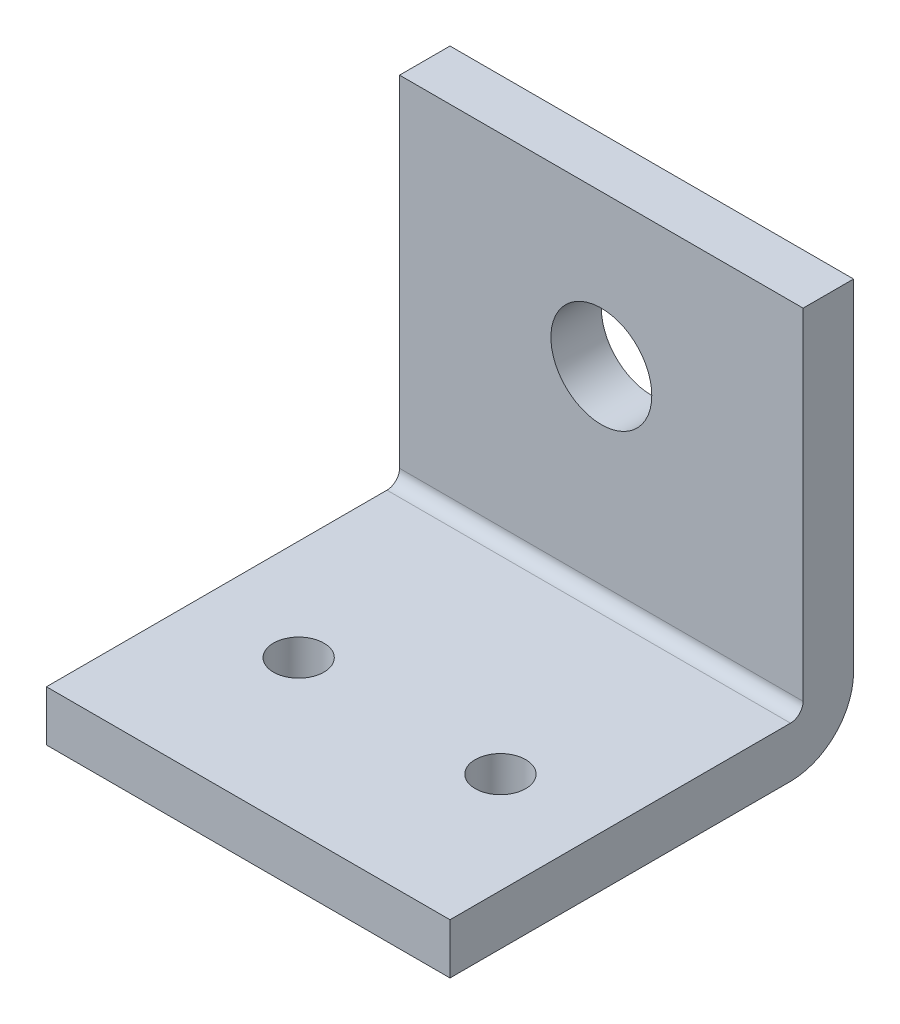
SolidWorks part; units mm, degrees
ref_plane "Front Plane" through (0, 0, 0) normal (0, 0, 1) x (1, 0, 0)
ref_plane "Top Plane" through (0, 0, 0) normal (0, 1, 0) x (1, 0, 0)
ref_plane "Right Plane" through (0, 0, 0) normal (1, 0, 0) x (0, 0, -1)
sketch "Sketch1" plane through (0, 0, 0) normal (1, 0, 0) x (0, 0, -1)
  line L0 (11.8056, 25.625) -> (11.8056, -8.125)
  line L1 (10.5556, -9.375) -> (-23.1944, -9.375)
  line L2 (-23.1944, -9.375) -> (-23.1944, -14.375)
  line L3 (-23.1944, -14.375) -> (10.5556, -14.375)
  line L4 (16.8056, -8.125) -> (16.8056, 25.625)
  line L5 (16.8056, 25.625) -> (11.8056, 25.625)
  arc A0 (16.8056, -8.125) -> (10.5556, -14.375) centre (10.5556, -8.125) cw
  arc A1 (11.8056, -8.125) -> (10.5556, -9.375) centre (10.5556, -8.125) cw
  point P8 (16.8056, -14.375)
  dimension "D5" = 6.25
  dimension "D6" = 1.25
  dimension "D1" = 5
  dimension "D2" = 5
  dimension "D3" = 40
  dimension "D4" = 40
extrude "Boss-Extrude1" add sketch "Sketch1" against normal blind 40
sketch "Sketch2" plane through (0, 0, -11.8056) normal (0, 0, 1) x (1, 0, 0)
  line L0 (-40, 25.625) -> (-40, -8.125) construction
  line L1 (-40, 25.625) -> (0, 25.625) construction
  circle A0 centre (-20, 10.625) radius 5
  dimension "D3" = 10
  dimension "D1" = 20
  dimension "D2" = 15
extrude "Cut-Extrude1" cut sketch "Sketch2" against normal blind 40
sketch "Sketch3" plane through (0, -9.375, 0) normal (0, 1, 0) x (1, 0, 0)
  line L0 (-45.0676, -8.1944) -> (7.7362, -8.1944) construction
  line L1 (-40, 10.5556) -> (-40, -23.1944) construction
  line L2 (-40, -23.1944) -> (0, -23.1944) construction
  circle A0 centre (-30, -8.1944) radius 2.5
  circle A1 centre (-10, -8.1944) radius 2.5
  dimension "D4" = 5
  dimension "D5" = 5
  dimension "D1" = 10
  dimension "D2" = 20
  dimension "D3" = 15
extrude "Cut-Extrude2" cut sketch "Sketch3" against normal blind 40
